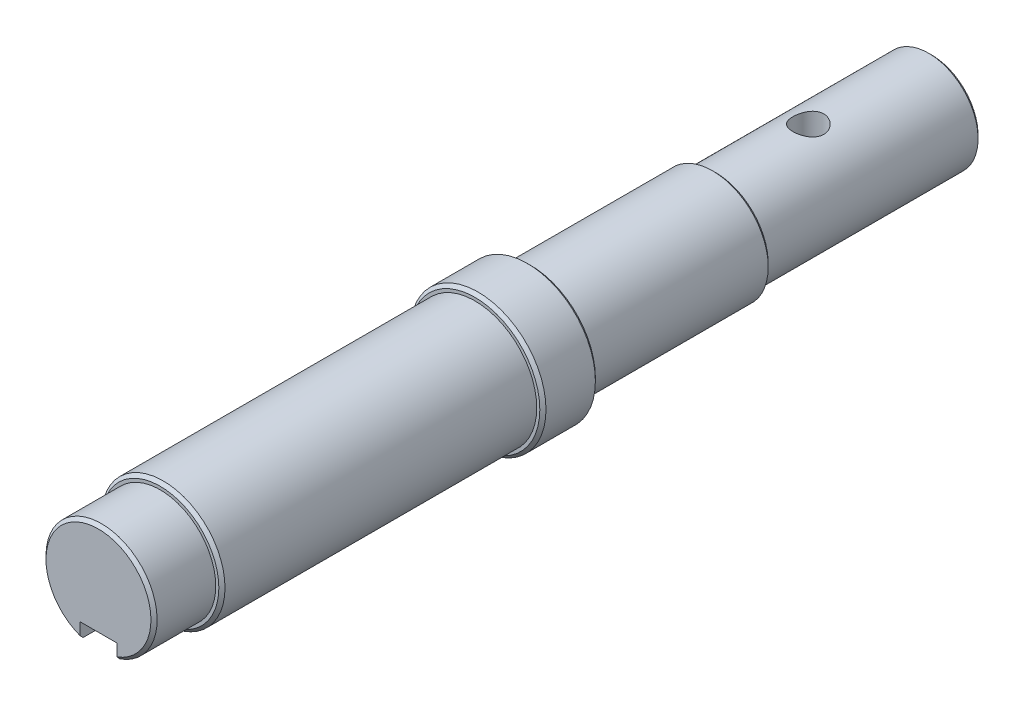
from build123d import *

# Parameters (mm, degrees)
SKETCH1_R           = 11
BOSS_EXTRUDE1_DEPTH = 4.5
SKETCH2_R           = 9
BOSS_EXTRUDE2_DEPTH = 30
SKETCH3_R           = 10
BOSS_EXTRUDE3_DEPTH = 51
BOSS_EXTRUDE4_START = 10
SKETCH4_R           = 9
BOSS_EXTRUDE4_DEPTH = 10
CUT_EXTRUDE1_DEPTH  = 15
BOSS_EXTRUDE5_DEPTH = 6
CUT_EXTRUDE2_DEPTH  = 19
BOSS_EXTRUDE6_DEPTH = 6
CHAMFER1_SIZE       = 0.5
SKETCH9_R           = 8
BOSS_EXTRUDE7_DEPTH = 35
CHAMFER2_SIZE       = 0.5
SKETCH10_R          = 2.5
CUT_EXTRUDE3_DEPTH  = 15


with BuildPart() as part:
    # Sketch1 → Boss-Extrude1 (new, symmetric)
    with BuildSketch(Plane.XY):
        Circle(SKETCH1_R)
    extrude(amount=BOSS_EXTRUDE1_DEPTH, both=True)

    # Sketch2 → Boss-Extrude2 (add)
    with BuildSketch(Plane(origin=(0, 0, -4.5), x_dir=(-1, 0, 0), z_dir=(0, 0, -1))):
        with Locations(Location((0, 0, 0), (0, 0, 180))):
            Circle(SKETCH2_R)
    extrude(amount=BOSS_EXTRUDE2_DEPTH)

    # Sketch3 → Boss-Extrude3 (add)
    with BuildSketch(Plane.XY.offset(4.5)):
        Circle(SKETCH3_R)
    extrude(amount=BOSS_EXTRUDE3_DEPTH)

    # Sketch4 → Boss-Extrude4 (add)
    with BuildSketch(Plane.XY.offset(55.5).offset(BOSS_EXTRUDE4_START)):
        Circle(SKETCH4_R)
    extrude(amount=-BOSS_EXTRUDE4_DEPTH)

    # Sketch5 → Cut-Extrude1 (cut)
    with BuildSketch(Plane(origin=(0, 0, 0), x_dir=(1, 0, 0), z_dir=(0, 1, 0))):
        with BuildLine():
            Line((-3, -65.5), (-3, -59.5))
            ThreePointArc((-3, -59.5), (0, -56.5), (3, -59.5))
            Line((3, -59.5), (3, -65.5))
            ThreePointArc((3, -65.5), (0, -68.5), (-3, -65.5))
        make_face()
    extrude(amount=-CUT_EXTRUDE1_DEPTH, mode=Mode.SUBTRACT)

    # Sketch6 → Boss-Extrude5 (add)
    with BuildSketch(Plane.XZ):
        with BuildLine():
            Line((3, 65.5), (-3, 65.5))
            Line((-3, 65.5), (-3, 59.5))
            ThreePointArc((-3, 59.5), (0, 56.5), (3, 59.5))
            Line((3, 59.5), (3, 65.5))
        make_face()
    extrude(amount=BOSS_EXTRUDE5_DEPTH)

    # Sketch7 → Cut-Extrude2 (cut)
    with BuildSketch(Plane(origin=(0, 0, 0), x_dir=(1, 0, 0), z_dir=(0, 1, 0))):
        with BuildLine():
            Line((3, 10.5), (3, 8.5))
            ThreePointArc((3, 8.5), (0, 5.5), (-3, 8.5))
            Line((-3, 8.5), (-3, 10.5))
            ThreePointArc((-3, 10.5), (0, 13.5), (3, 10.5))
        make_face()
    extrude(amount=-CUT_EXTRUDE2_DEPTH, mode=Mode.SUBTRACT)

    # Sketch8 → Boss-Extrude6 (add)
    with BuildSketch(Plane.XZ):
        with BuildLine():
            Line((3, -10.5), (3, -8.5))
            ThreePointArc((3, -8.5), (0, -5.5), (-3, -8.5))
            Line((-3, -8.5), (-3, -10.5))
            ThreePointArc((-3, -10.5), (0, -13.5), (3, -10.5))
        make_face()
    extrude(amount=BOSS_EXTRUDE6_DEPTH)

    # Chamfer1
    chamfer1_edges = [part.edges().sort_by_distance(p)[0] for p in [
        (-10, 0, 55.5),
        (-5.196152423, 7.348469228, 65.5),
        (-11, 0, -4.5),
        (-11, 0, 4.5),
        (-9, 0, -34.5),
    ]]
    chamfer(chamfer1_edges, length=CHAMFER1_SIZE)

    # Sketch9 → Boss-Extrude7 (add)
    with BuildSketch(Plane(origin=(0, 0, -34.5), x_dir=(-1, 0, 0), z_dir=(0, 0, -1))):
        Circle(SKETCH9_R)
    extrude(amount=BOSS_EXTRUDE7_DEPTH)

    # Chamfer2
    chamfer2_edges = [part.edges().sort_by_distance(p)[0] for p in [
        (8, 0, -69.5),
    ]]
    chamfer(chamfer2_edges, length=CHAMFER2_SIZE)

    # Sketch10 → Cut-Extrude3 (cut, symmetric)
    with BuildSketch(Plane(origin=(0, 0, 0), x_dir=(1, 0, 0), z_dir=(0, 1, 0))):
        with Locations(Location((0, 49.5, 0), (0, 0, 270))):
            Circle(SKETCH10_R)
    extrude(amount=CUT_EXTRUDE3_DEPTH, both=True, mode=Mode.SUBTRACT)


solid = part.part
